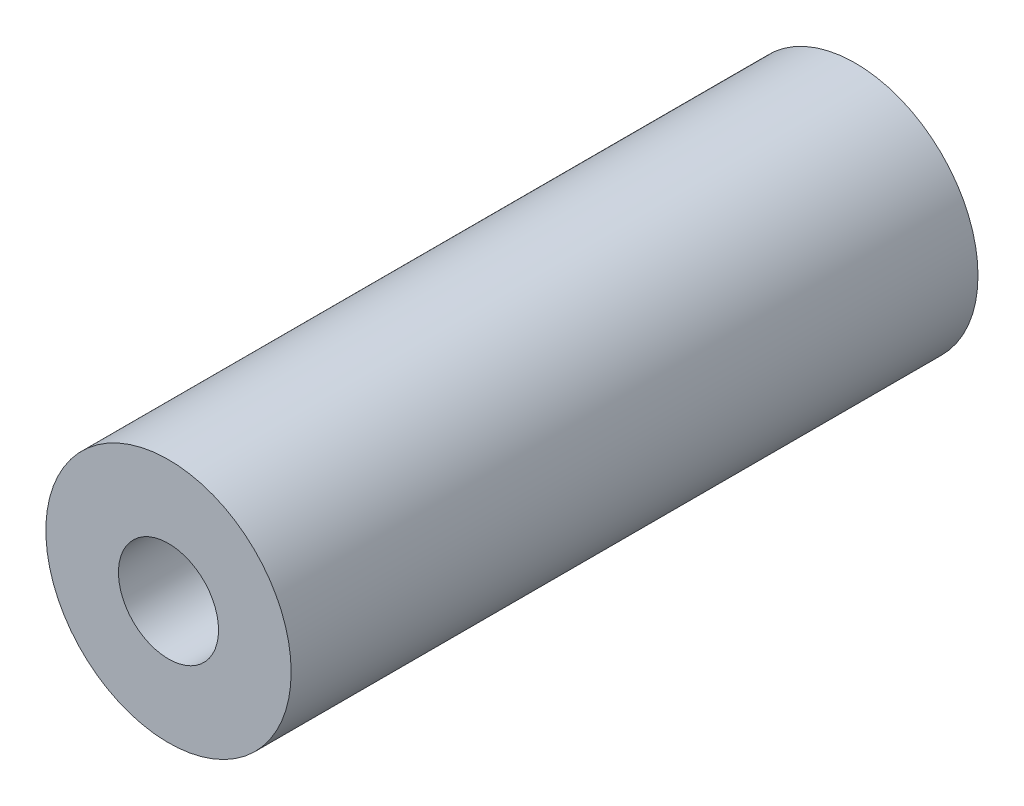
SolidWorks part; units mm, degrees
material "AISI 1045 钢，冷拔"
ref_plane "Front Plane" through (0, 0, 0) normal (0, 0, 1) x (1, 0, 0)
ref_plane "Top Plane" through (0, 0, 0) normal (0, 1, 0) x (1, 0, 0)
ref_plane "Right Plane" through (0, 0, 0) normal (1, 0, 0) x (0, 0, -1)
sketch "Sketch1" plane through (0, 0, 0) normal (0, 0, 1) x (1, 0, 0)
  circle A0 centre (0, 0) radius 12.5
  dimension "D1" = 25
extrude "Boss-Extrude1" add sketch "Sketch1" along normal blind 70
hole_wizard "M12 Tapped Hole1" positions "Sketch3" profile "Sketch2" tap size "M12" standard "Iso"
sketch "Sketch3" plane through (0, 0, 70) normal (0, 0, 1) x (1, 0, 0)
  point P0 (0, 0)
sketch "Sketch2" plane through (0, 0, 70) normal (1, 0, 0) x (0, -1, 0)
  line L0 (0, 0) -> (0, 33.0644)
  line L1 (0, 33.0644) -> (5.1, 30)
  line L2 (5.1, 30) -> (5.1, 0)
  line L5 (5.1, 0) -> (0, 0)
  line L10 (0, 33.0644) -> (-5.1, 30) construction
  line L11 (0, -6.35) -> (0, 107.95) construction
  dimension "螺纹孔钻头直径" = 10.2
  dimension "螺纹孔钻头深度" = 30
  dimension "导头角度" = 118
cosmetic thread "Cosmetic thread1" parameters "D1"=30, "D2"=12
hole_wizard "M12 Tapped Hole2" positions "Sketch5" profile "Sketch4" tap size "M12" standard "Iso"
sketch "Sketch5" plane through (0, 0, 0) normal (0, 0, -1) x (-1, 0, 0)
  point P0 (0, 0)
sketch "Sketch4" plane through (0, 0, 0) normal (1, 0, 0) x (0, 1, 0)
  line L0 (0, 0) -> (0, 33.0644)
  line L1 (0, 33.0644) -> (5.1, 30)
  line L2 (5.1, 30) -> (5.1, 0)
  line L5 (5.1, 0) -> (0, 0)
  line L10 (0, 33.0644) -> (-5.1, 30) construction
  line L11 (0, -6.35) -> (0, 107.95) construction
  dimension "螺纹孔钻头直径" = 10.2
  dimension "螺纹孔钻头深度" = 30
  dimension "导头角度" = 118
cosmetic thread "Cosmetic thread2" parameters "D1"=30, "D2"=12
